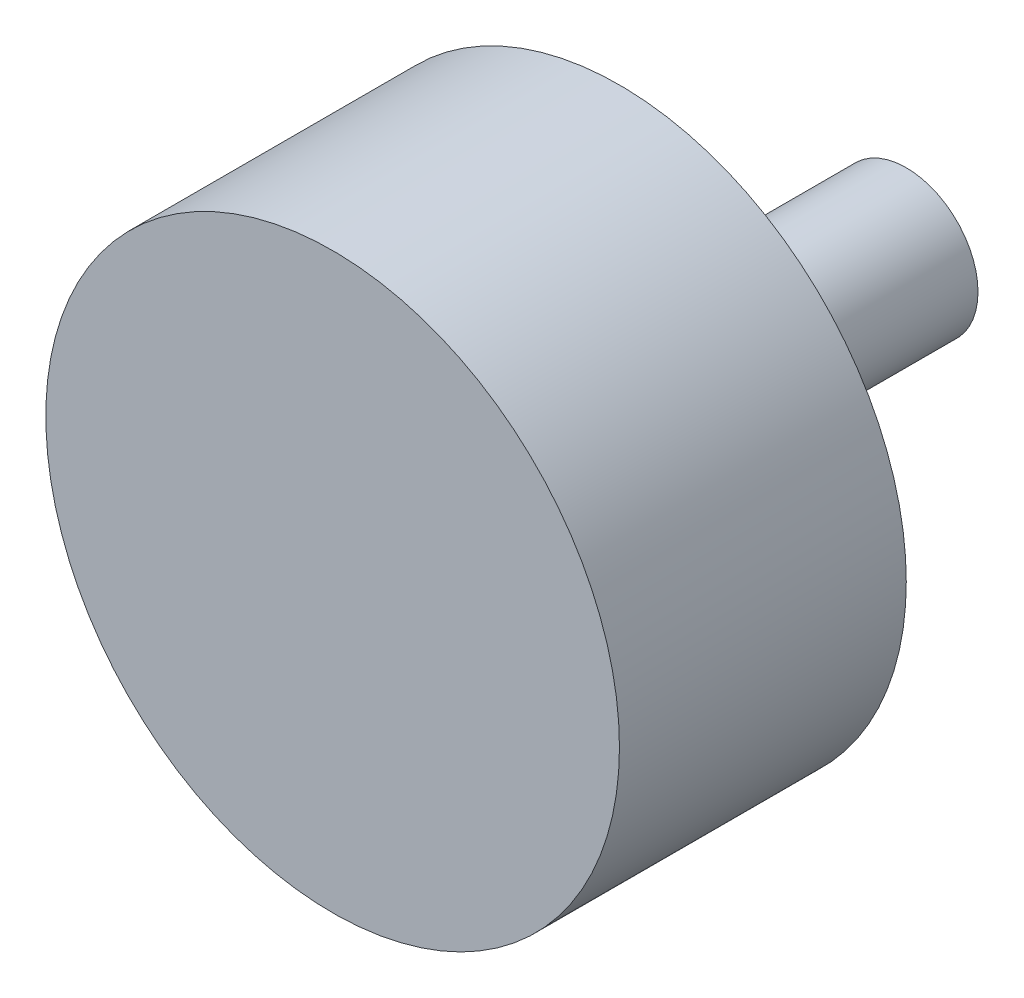
SolidWorks part; units mm, degrees
ref_plane "Front Plane" through (0, 0, 0) normal (0, 0, 1) x (1, 0, 0)
ref_plane "Top Plane" through (0, 0, 0) normal (0, 1, 0) x (1, 0, 0)
ref_plane "Right Plane" through (0, 0, 0) normal (1, 0, 0) x (0, 0, -1)
other "Configuration Table"
sketch "Sketch1" plane through (0, 0, 0) normal (0, 0, 1) x (1, 0, 0)
  circle A0 centre (0, 0) radius 2.5
  dimension "D1" = 5
extrude "Boss-Extrude1" add sketch "Sketch1" along normal blind 10
sketch "Sketch2" plane through (0, 0, 10) normal (0, 0, 1) x (1, 0, 0)
  circle A0 centre (0, 0) radius 10
  dimension "D1" = 20
extrude "Boss-Extrude2" add sketch "Sketch2" along normal blind 10
